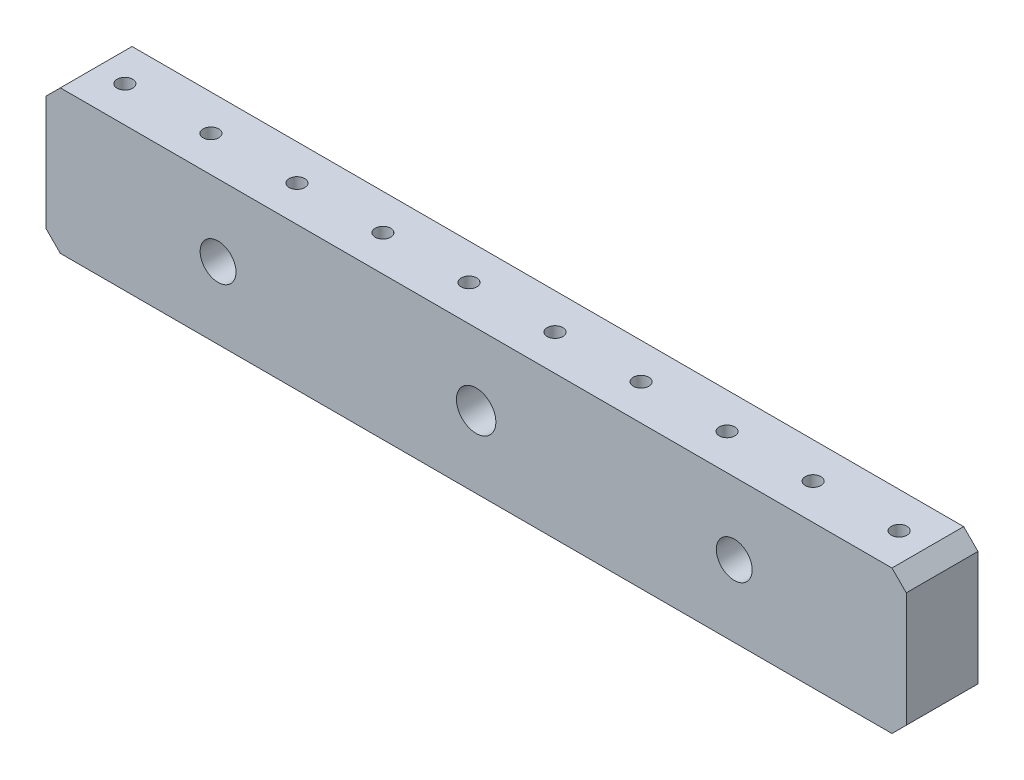
from build123d import *

# Parameters (mm, degrees)
SKETCH_1_W             = 120
SKETCH_1_H             = 10
EXTRUDE_1_DEPTH        = 20
SKETCH_2_R             = 1.09
CUT_EXTRUDE_1_DEPTH    = 3
SKETCH_4_R             = 0.825
CUT_EXTRUDE_2_DEPTH    = 30
PATTERN_LINEAR_1_COUNT = 10
PATTERN_LINEAR_1_PITCH = 12
CHAMFER_1_SIZE         = 2
MM_1_D                 = 5
MM_1_DEPTH             = 15
MM_1_TIP               = 1.502151548
HOLE_WIZARD_M5_1_D     = 5.5
HOLE_WIZARD_M5_1_DEPTH = 15
HOLE_WIZARD_M5_1_TIP   = 1.652366702


with BuildPart() as part:
    # 草图1 → 凸台-拉伸1 (new body)
    with BuildSketch(Plane(origin=(0, 0, 0), x_dir=(1, 0, 0), z_dir=(0, 1, 0))):
        Rectangle(SKETCH_1_W, SKETCH_1_H)
    extrude(amount=EXTRUDE_1_DEPTH)

    # 草图2 → 切除-拉伸1 (cut)
    with BuildSketch(Plane(origin=(0, 20, 0), x_dir=(1, 0, 0), z_dir=(0, 1, 0))):
        with Locations(Location((-54, 0, 0), (0, 0, 270))):
            Circle(SKETCH_2_R)
    cut_extrude_1 = extrude(amount=-CUT_EXTRUDE_1_DEPTH, mode=Mode.SUBTRACT)

    # 草图4 → 切除-拉伸2 (cut)
    with BuildSketch(Plane(origin=(0, 17, 0), x_dir=(1, 0, 0), z_dir=(0, 1, 0))):
        with Locations(Location((-54, 0, 0), (0, 0, 270))):
            Circle(SKETCH_4_R)
    cut_extrude_2 = extrude(amount=-CUT_EXTRUDE_2_DEPTH, mode=Mode.SUBTRACT)

    # 阵列(线性)1: 切除-拉伸1, 切除-拉伸2 ×10
    with Locations(*[(i * PATTERN_LINEAR_1_PITCH, 0, 0) for i in range(1, PATTERN_LINEAR_1_COUNT)]):
        add(cut_extrude_1, mode=Mode.SUBTRACT)
        add(cut_extrude_2, mode=Mode.SUBTRACT)

    # 倒角1
    chamfer_1_edges = [part.edges().sort_by_distance(p)[0] for p in [
        (-60, 20, 0),
        (60, 20, 0),
        (-60, 0, 0),
        (60, 0, 0),
    ]]
    chamfer(chamfer_1_edges, length=CHAMFER_1_SIZE)

    # 大小mm 暗销孔1
    with Locations(Plane.XY.offset(5)):
        with Locations((36, 10), (-36, 10)):
            Hole(MM_1_D / 2, depth=MM_1_DEPTH)
            with Locations((0, 0, -(MM_1_DEPTH + MM_1_TIP / 2))):  # 118° drill point
                Cone(0, MM_1_D / 2, MM_1_TIP, mode=Mode.SUBTRACT)

    # M5 间隙孔1
    with Locations(Plane.XY.offset(5)):
        with Locations((0, 10)):
            Hole(HOLE_WIZARD_M5_1_D / 2, depth=HOLE_WIZARD_M5_1_DEPTH)
            with Locations((0, 0, -(HOLE_WIZARD_M5_1_DEPTH + HOLE_WIZARD_M5_1_TIP / 2))):  # 118° drill point
                Cone(0, HOLE_WIZARD_M5_1_D / 2, HOLE_WIZARD_M5_1_TIP, mode=Mode.SUBTRACT)


solid = part.part
